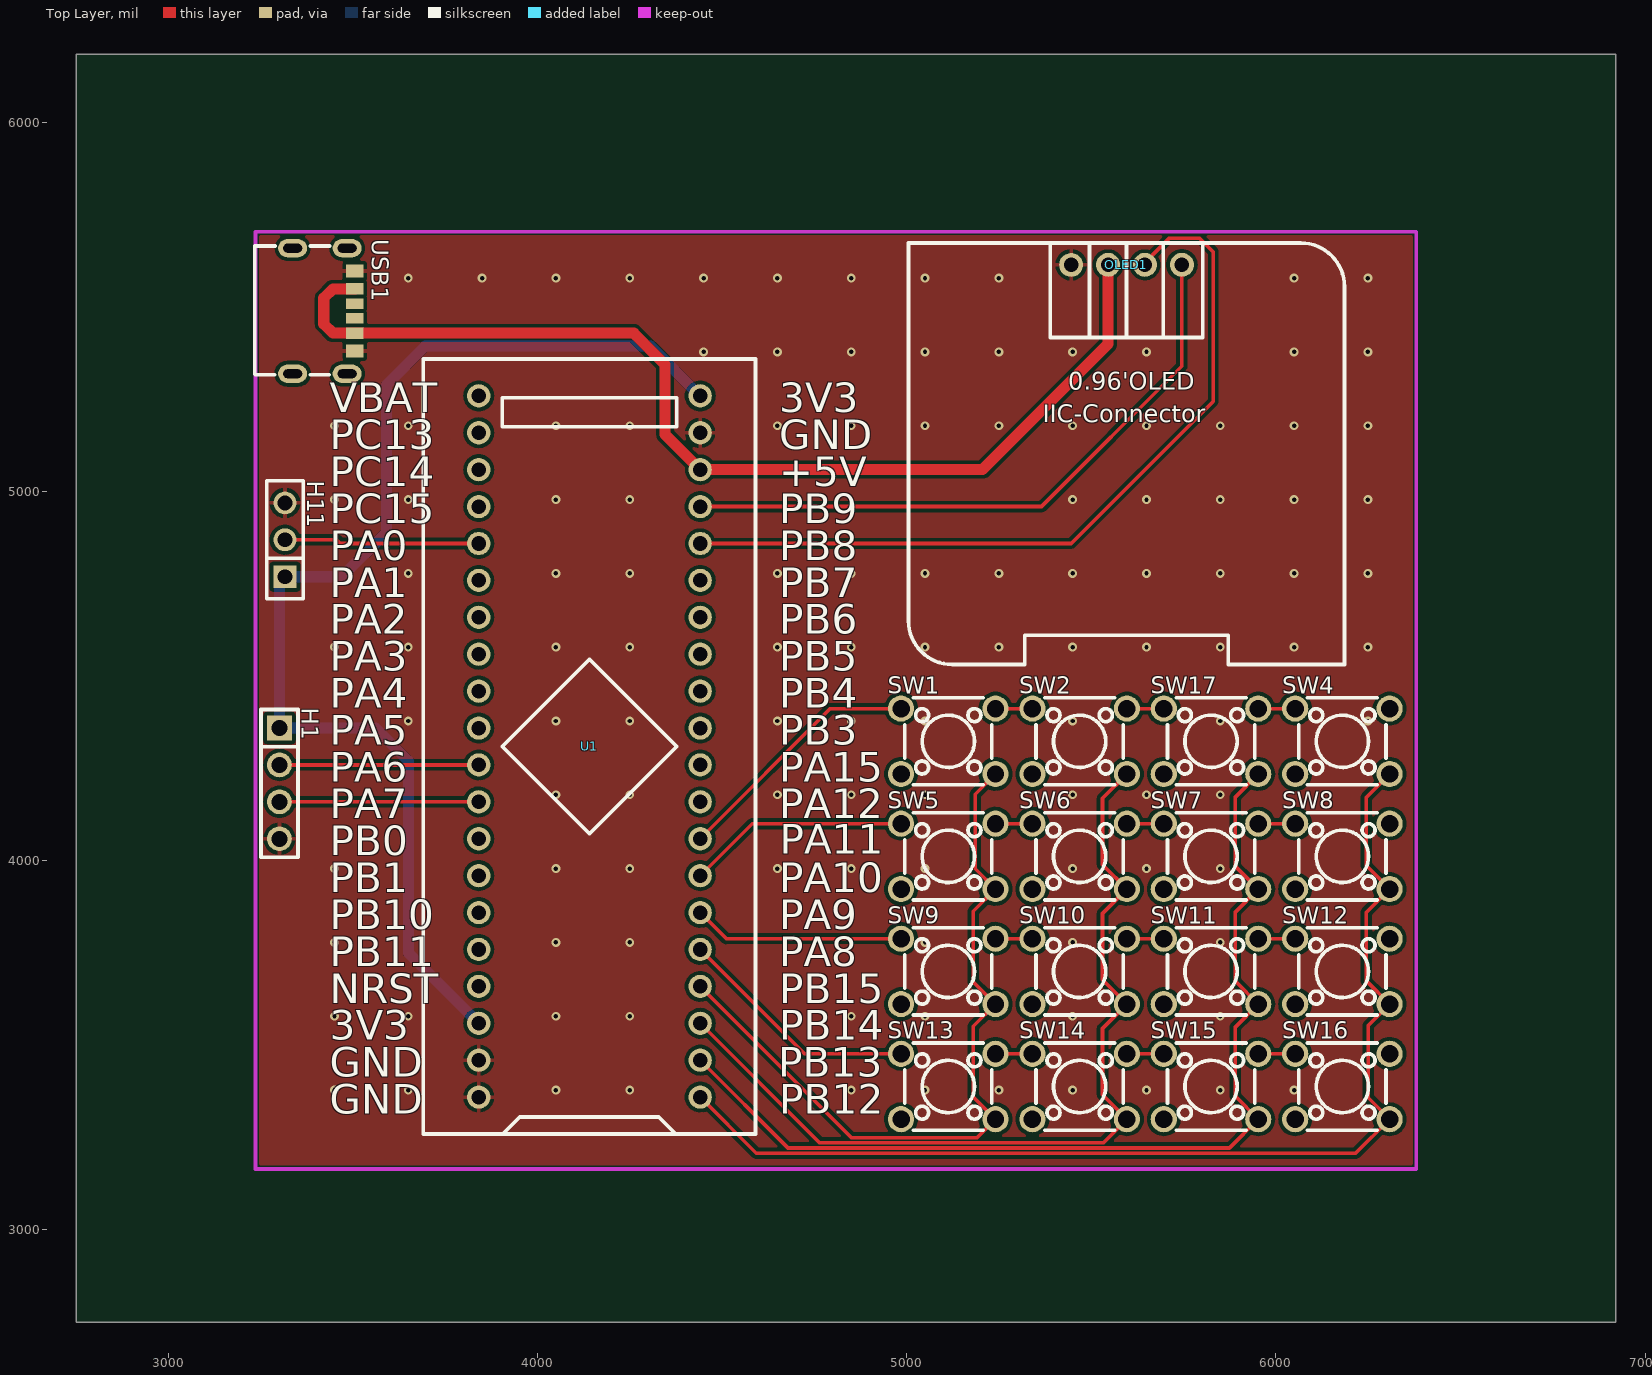
[diagram p0: Top Layer view]
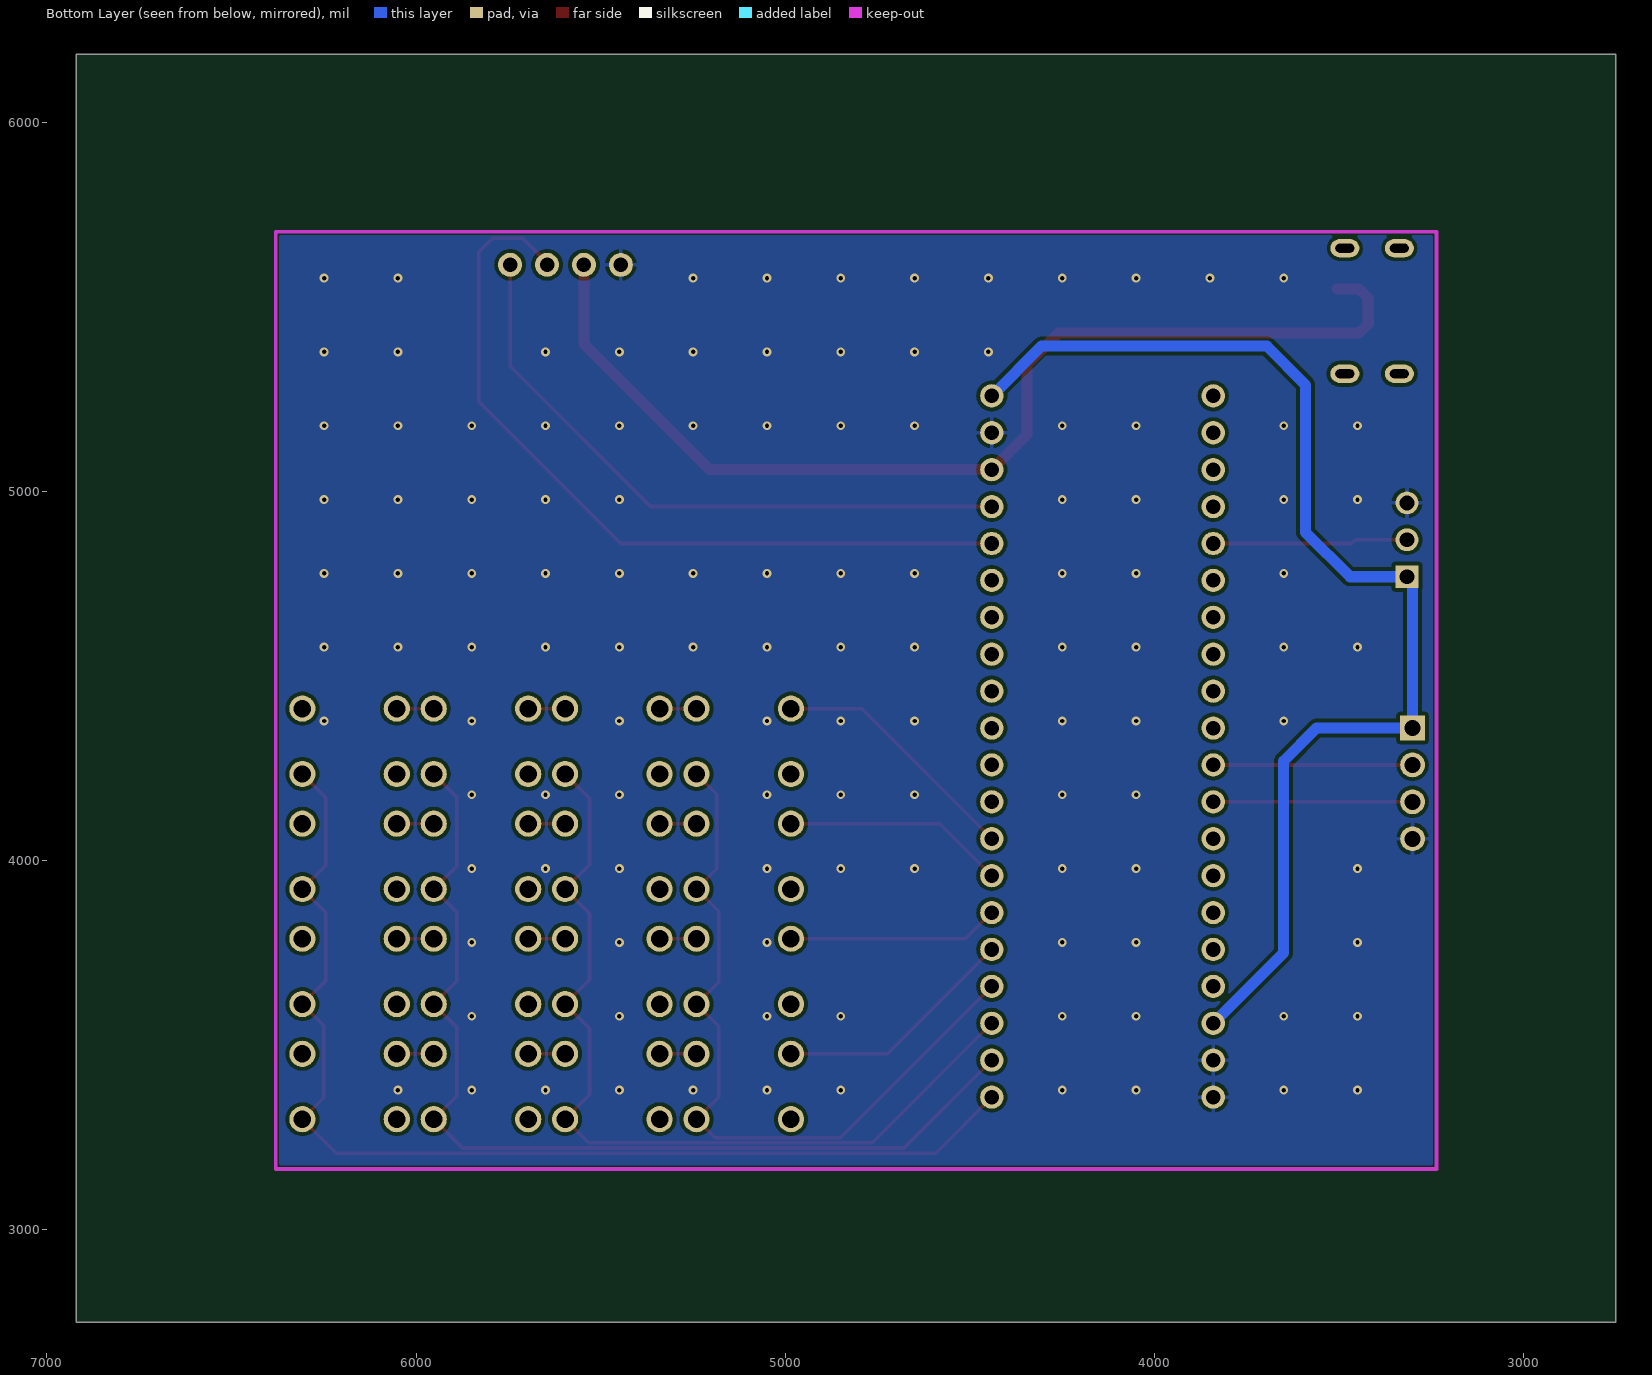
[diagram p1: Bottom Layer view, seen from below]
# Altium PCB MISC51803.pcbdoc
Units mil, origin at the board's own origin, x right, y up, seen from the top; angles counter-clockwise.
Board outline 4170 x 3435 mil, 2 copper layers (Top Layer, Bottom Layer), stack 62.206 mil thick; 21 components, 49 nets, 125 pads, 118 vias.

## Layer stack, top to bottom
Top Solder Mask Layer: solder mask 0.394, Dk 3.3
Top Layer: signal copper 1.379
Dielectric1: surface 59.449, FR4, Dk 4.5
Bottom Layer: signal copper 1.378
Bottom Solder Mask Layer: solder mask 0.394, Dk 3.3

## Board outline
6920,2750 2750,2750 2750,6185 6920,6185

## Design rules (kind name [scope] priority, off if disabled: settings)
BoardOutlineClearance copperThickness2oz_1 [All] p2 off: genericclearance=7.99 ignorepadtopadclearanceinfootprint=FALSE except(0: Arc-SplitContinuation Track-SplitContinuation SMDPad-SplitContinuation THPad-SplitContinuation Via-SplitContinuation Fill-SplitContinuation Region-SplitContinuation Poly-SplitContinuation Text-SplitContinuation Hole-SplitContinuation; 5.98: Arc-CutoutEdge SMDPad-CutoutEdge THPad-CutoutEdge Via-CutoutEdge Fill-CutoutEdge Region-CutoutEdge Text-CutoutEdge; 6.93: Hole-OutlineEdge Hole-CutoutEdge; 10: Poly-OutlineEdge Poly-CutoutEdge; 11.81: Arc-OutlineEdge Track-OutlineEdge SMDPad-OutlineEdge THPad-OutlineEdge Via-OutlineEdge Fill-OutlineEdge Region-OutlineEdge Text-OutlineEdge Track-CutoutEdge)
BoardOutlineClearance copperThickness1oz_1 [All] p4: genericclearance=4.02 ignorepadtopadclearanceinfootprint=FALSE except(0: Arc-SplitContinuation Track-SplitContinuation SMDPad-SplitContinuation THPad-SplitContinuation Via-SplitContinuation Fill-SplitContinuation Region-SplitContinuation Poly-SplitContinuation Text-SplitContinuation Hole-SplitContinuation; 6: SMDPad-CutoutEdge THPad-CutoutEdge Via-CutoutEdge Fill-CutoutEdge Region-CutoutEdge Text-CutoutEdge; 6.93: Hole-OutlineEdge Hole-CutoutEdge; 10: Poly-OutlineEdge Poly-CutoutEdge; 11.8: Arc-OutlineEdge Track-OutlineEdge SMDPad-OutlineEdge THPad-OutlineEdge Via-OutlineEdge Fill-OutlineEdge Region-OutlineEdge Text-OutlineEdge; 11.81: Arc-CutoutEdge Track-CutoutEdge)
Clearance copperThickness2oz [All] p1 off: gap=7.99 ignorepadtopadclearanceinfootprint=FALSE except(5.98: SMDPad-Track SMDPad-SMDPad THPad-Track SMDPad-THPad THPad-THPad Track-Via SMDPad-Via THPad-Via Via-Via Fill-Track Region-Track Fill-SMDPad Region-SMDPad Fill-THPad Region-THPad Fill-Via Region-Via Fill-Fill Fill-Region Region-Region Arc-Track Arc-SMDPad Arc-THPad Arc-Via Fill-Arc Region-Arc Arc-Arc Text-Track SMDPad-Text Text-THPad Text-Via Fill-Text Region-Text Arc-Text Text-Text; 6.93: Hole-Track Hole-SMDPad Hole-THPad Hole-Via Fill-Hole Region-Hole Hole-Arc Hole-Text; 10: Poly-Track Poly-SMDPad Poly-THPad Poly-Via Poly-Fill Poly-Region Poly-Poly Poly-Arc Poly-Text Poly-Hole)
Clearance copperThickness1oz [All] p3: gap=4.02 ignorepadtopadclearanceinfootprint=FALSE except(5.98: SMDPad-Track SMDPad-SMDPad THPad-Track SMDPad-THPad THPad-THPad Track-Via SMDPad-Via THPad-Via Via-Via Fill-Track Region-Track Fill-SMDPad Region-SMDPad Fill-THPad Region-THPad Fill-Via Region-Via Fill-Fill Fill-Region Region-Region; 6: Arc-Track Arc-SMDPad Arc-THPad Arc-Via Fill-Arc Region-Arc Arc-Arc Text-Track SMDPad-Text Text-THPad Text-Via Fill-Text Region-Text Arc-Text Text-Text; 6.93: Hole-Track Hole-SMDPad Hole-THPad Hole-Via Fill-Hole Region-Hole Hole-Arc Hole-Text; 10: Poly-Track Poly-SMDPad Poly-THPad Poly-Via Poly-Fill Poly-Region Poly-Poly Poly-Arc Poly-Text Poly-Hole)
DiffPairsRouting differentialPair [All] p1: maxlimit=6 minlimit=6 mostfreqgap=6 toplayer_minwidth=5 toplayer_prefwidth=10 toplayer_maxwidth=100 toplayer_mingap=6 toplayer_prefgap=6 toplayer_maxgap=6 bottomlayer_minwidth=5 bottomlayer_prefwidth=10 bottomlayer_maxwidth=100 bottomlayer_mingap=6 bottomlayer_prefgap=6 bottomlayer_maxgap=6 maxuncoupledlength=10
HoleToHoleClearance otherClearance [All] p1: gap=11.81 allowstackedmicrovias=TRUE
Length netLength [All] p1: minlimit=0 maxlimit=0
MatchedLengths netLengthTolerance [All] p1: tolerance=1000
PasteMaskExpansion pasteMaskExpansion [All] p1: expansion=0
PlaneConnect innerPlane [All] p1: planeconnectstyle=Relief reliefexpansion=20 reliefentries=4 reliefconductorwidth=10 reliefairgap=10
PolygonConnect copperRegion [(InNet('GND'))] p1: connectstyle=Relief reliefconductorwidth=10 reliefentries=4 polygonreliefangle="90 Angle" airgapwidth=10 via.connectstyle=Relief via.reliefconductorwidth=10 via.reliefentries=4 via.polygonreliefangle="90 Angle" via.airgapwidth=10
RoutingVias viaSize [All] p1: holewidth=12.01 width=24.02 viastyle="Through Hole" minholewidth=11.81 minwidth=19.68 maxholewidth=248.03 maxwidth=393.7
SolderMaskExpansion solderMaskExpansion [IsVia] p1: expansion=-1000 istentingtop=TRUE
SolderMaskExpansion solderMaskExpansion [All] p2: expansion=2 istentingtop=FALSE
Width copperThickness2oz_2 [All] p1 off: maxlimit=100 minlimit=8 preferedwidth=10
Width copperThickness1oz_2 [All] p2: maxlimit=100 minlimit=5 preferedwidth=10

## Components (designator, comment, footprint, x,y, rotation, side; value= is the part's Value field where it differs from the comment)
H1 "" HDR-TH_4P-P2.54-V-M 3300,4210 r270 top
H11 "" HDR-TH_3P-P2.54-V-F 3315,4870 r90 top
OLED1 "" 0.96OLED_4P 5595,5615 r0 top
SW1 "KH-6X6X6H-TJ" SW-TH_4P-L6.0-W6.0-P4.50-LS6.5 5112.09,4324.04 r0 top
SW2 "KH-6X6X6H-TJ" SW-TH_4P-L6.0-W6.0-P4.50-LS6.5 5468.06,4324.04 r0 top
SW4 "KH-6X6X6H-TJ" SW-TH_4P-L6.0-W6.0-P4.50-LS6.5 6180,4324.04 r0 top
SW5 "KH-6X6X6H-TJ" SW-TH_4P-L6.0-W6.0-P4.50-LS6.5 5112.09,4012.26 r0 top
SW6 "KH-6X6X6H-TJ" SW-TH_4P-L6.0-W6.0-P4.50-LS6.5 5468.06,4012.26 r0 top
SW7 "KH-6X6X6H-TJ" SW-TH_4P-L6.0-W6.0-P4.50-LS6.5 5824.03,4012.26 r0 top
SW8 "KH-6X6X6H-TJ" SW-TH_4P-L6.0-W6.0-P4.50-LS6.5 6180,4012.26 r0 top
SW9 "KH-6X6X6H-TJ" SW-TH_4P-L6.0-W6.0-P4.50-LS6.5 5112.09,3700.49 r0 top
SW10 "KH-6X6X6H-TJ" SW-TH_4P-L6.0-W6.0-P4.50-LS6.5 5468.06,3700.49 r0 top
SW11 "KH-6X6X6H-TJ" SW-TH_4P-L6.0-W6.0-P4.50-LS6.5 5824.03,3700.49 r0 top
SW12 "KH-6X6X6H-TJ" SW-TH_4P-L6.0-W6.0-P4.50-LS6.5 6180,3700.49 r0 top
SW13 "KH-6X6X6H-TJ" SW-TH_4P-L6.0-W6.0-P4.50-LS6.5 5112.09,3388.72 r0 top
SW14 "KH-6X6X6H-TJ" SW-TH_4P-L6.0-W6.0-P4.50-LS6.5 5468.06,3388.72 r0 top
SW15 "KH-6X6X6H-TJ" SW-TH_4P-L6.0-W6.0-P4.50-LS6.5 5824.03,3388.72 r0 top
SW16 "KH-6X6X6H-TJ" SW-TH_4P-L6.0-W6.0-P4.50-LS6.5 6180,3388.72 r0 top
SW17 "KH-6X6X6H-TJ" SW-TH_4P-L6.0-W6.0-P4.50-LS6.5 5824.03,4324.04 r0 top
U1 "STM32F103C8T6-Card" CONN-TH_L53.3-W22.9_STM32F103C8T6-CARD 4140,4310 r90 top
USB1 "" "USB_ TYPE-C-6P" 3420,5495 r270 top

## Footprints (in the part's own frame and the unit in brackets; to place one, negate y for a bottom-side part, rotate by r counter-clockwise, add the part's x,y. Pads: shape width x height; smd on the part's side, far side on the other; paste and mask are expansions set on the pad)
0.96OLED_4P [mm]
  round 1.65 hole 1 copper offset 0,0: 1(-3.81,-0.001) 2(-1.27,0.002) 3(1.27,0.002) 4(3.81,0.002)
  silkscreen extent -15,-27.5 15,1.5
CONN-TH_L53.3-W22.9_STM32F103C8T6-CARD [mm]
  round 1.6 hole 1: 1(-24.13,-7.62) 2(-21.59,-7.62) 3(-19.05,-7.62) 4(-16.51,-7.62) 5(-13.97,-7.62) 6(-11.43,-7.62) 7(-8.89,-7.62) 8(-6.35,-7.62) 9(-3.81,-7.62) 10(-1.27,-7.62) 11(1.27,-7.62) 12(3.81,-7.62) 13(6.35,-7.62) 14(8.89,-7.62) 15(11.43,-7.62) 16(13.97,-7.62) 17(16.51,-7.62) 18(19.05,-7.62) 19(21.59,-7.62) 20(24.13,-7.62) 21(24.13,7.62) 22(21.59,7.62) 23(19.05,7.62) 24(16.51,7.62) 25(13.97,7.62) 26(11.43,7.62) 27(8.89,7.62) 28(6.35,7.62) 29(3.81,7.62) 30(1.27,7.62) 31(-1.27,7.62) 32(-3.81,7.62) 33(-6.35,7.62) 34(-8.89,7.62) 35(-11.43,7.62) 36(-13.97,7.62) 37(-16.51,7.62) 38(-19.05,7.62) 39(-21.59,7.62) 40(-24.13,7.62)
  silkscreen extent -26.67,-11.43 26.67,11.43
HDR-TH_3P-P2.54-V-F [mil]
  rect 62x62 hole 40.16: 1(-100,0)
  round 62 hole 40.16: 2(0,0) 3(100,0)
  silkscreen extent -160,-49 160,49
HDR-TH_4P-P2.54-V-M [mm]
  rect 1.7x1.7 hole 1.1: 1(-3.81,0)
  round 1.7 hole 1.1: 2(-1.27,0) 3(1.27,0) 4(3.81,0)
  silkscreen extent -5.08,-1.27 5.08,1.27
SW-TH_4P-L6.0-W6.0-P4.50-LS6.5 [mm]
  round 1.8 hole 1.2: 1(-3.25,2.25) 2(3.25,2.25) 3(-3.25,-2.25) 4(3.25,-2.25)
  silkscreen extent -3,-3 3,3
"USB_ TYPE-C-6P" [mm]
  oval 1.25x2 hole 0.6 slot 1.3 at 90 deg paste+0 mask+0.05: 7(-4.193,1.611) 8(4.447,1.611) 9(-4.193,-2.139) 10(4.447,-2.139)
  rect 0.7x1.2 smd paste-100 mask+0.05: A5(-0.373,2.139) B5(0.627,2.139)
  rect 0.8x1.2 smd paste-100 mask+0.05: A9(1.647,2.139) B9(-1.393,2.139)
  rect 0.9x1.2 smd paste-100 mask+0.05: A12(2.877,2.139) B12(-2.623,2.139)
  silkscreen extent -4.34,-4.75 4.52,0.39

## Via types
v1: diameter 24.02, hole 12, Top Layer to Bottom Layer, 118 vias

## Nets (pads, with @x,y where several pads share a name; then routed paths per layer and width w, separated by ;. In a path a pad name is that pad's centre, name@x,y a point inside that pad or via, vN(x,y) a via of type N, cw(c..) or ccw(c..) an arc to the next point about the centre after c; other vN are vias at no path point)
$1N9: SW9.2 SW10.1 | length 100.1
  Top Layer w10: SW9.2 SW10.1
$1N10: SW13.2 SW14.1 | length 100.1
  Top Layer w10: SW13.2 SW14.1
$1N11: SW15.2 SW16.1 | length 100.1
  Top Layer w10: SW15.2 SW16.1
$1N12: SW14.2 SW15.1 | length 100.1
  Top Layer w10: SW14.2 SW15.1
$1N13: SW11.2 SW12.1 | length 100.1
  Top Layer w10: SW11.2 SW12.1
$1N14: SW10.2 SW11.1 | length 100.1
  Top Layer w10: SW10.2 SW11.1
$1N15: SW7.2 SW8.1 | length 100.1
  Top Layer w10: SW7.2 SW8.1
$1N16: SW5.2 SW6.1 | length 100.1
  Top Layer w10: SW5.2 SW6.1
$1N17: SW6.2 SW7.1 | length 100.1
  Top Layer w10: SW6.2 SW7.1
$1N18: SW1.2 SW2.1 | length 100.1
  Top Layer w10: SW1.2 SW2.1
$1N19: SW2.2 SW17.1 | length 100.1
  Top Layer w10: SW2.2 SW17.1
$1N20: SW4.1 SW17.2 | length 100.1
  Top Layer w10: SW17.2 SW4.1
+5V: OLED1.2 U1.18 USB1.A9 USB1.B9 | length 2920.3
  Top Layer w30: USB1.B9 3444.84,5549.84 3420,5525 3420,5455 3444.84,5430.16 USB1.A9 4259.84,5430.16 4345,5345 4345,5155 U1.18 5205,5060 5545,5400 OLED1.2@5545,5615.05
GND: H1.4 H11.3 OLED1.1 U1.19 U1.39 U1.40 USB1.A12 USB1.B12
  other v1: 3449.1,3379.1 3649.1,3379.1 4049.1,3379.1 4249.1,3379.1 4849.1,3379.1 5049.1,3379.1 5249.1,3379.1 5449.1,3379.1 5649.1,3379.1 5849.1,3379.1 6049.1,3379.1 3449.1,3579.1 3649.1,3579.1 4049.1,3579.1 4249.1,3579.1 4849.1,3579.1 5049.1,3579.1 5449.1,3579.1 5849.1,3579.1 3449.1,3779.1 4049.1,3779.1 4249.1,3779.1 5049.1,3779.1 5449.1,3779.1 5849.1,3779.1 3449.1,3979.1 4049.1,3979.1 4249.1,3979.1 4649.1,3979.1 4849.1,3979.1 5049.1,3979.1 5449.1,3979.1 5649.1,3979.1 5849.1,3979.1 4049.1,4179.1 4249.1,4179.1 4649.1,4179.1 4849.1,4179.1 5049.1,4179.1 5449.1,4179.1 5649.1,4179.1 5849.1,4179.1 3649.1,4379.1 4049.1,4379.1 4249.1,4379.1 4649.1,4379.1 4849.1,4379.1 5049.1,4379.1 5449.1,4379.1 5849.1,4379.1 6249.1,4379.1 3449.1,4579.1 3649.1,4579.1 4049.1,4579.1 4249.1,4579.1 4649.1,4579.1 4849.1,4579.1 5049.1,4579.1 5249.1,4579.1 5449.1,4579.1 5649.1,4579.1 5849.1,4579.1 6049.1,4579.1 6249.1,4579.1 3649.1,4779.1 4049.1,4779.1 4249.1,4779.1 4649.1,4779.1 4849.1,4779.1 5049.1,4779.1 5249.1,4779.1 5449.1,4779.1 5649.1,4779.1 5849.1,4779.1 6049.1,4779.1 6249.1,4779.1 3449.1,4979.1 3649.1,4979.1 4049.1,4979.1 4249.1,4979.1 5449.1,4979.1 5649.1,4979.1 5849.1,4979.1 6049.1,4979.1 6249.1,4979.1 3449.1,5179.1 3649.1,5179.1 4049.1,5179.1 4249.1,5179.1 4649.1,5179.1 4849.1,5179.1 5049.1,5179.1 5249.1,5179.1 5449.1,5179.1 5649.1,5179.1 5849.1,5179.1 6049.1,5179.1 6249.1,5179.1 4449.1,5379.1 4649.1,5379.1 4849.1,5379.1 5049.1,5379.1 5249.1,5379.1 5449.1,5379.1 5649.1,5379.1 6049.1,5379.1 6249.1,5379.1 3649.1,5579.1 3849.1,5579.1 4049.1,5579.1 4249.1,5579.1 4449.1,5579.1 4649.1,5579.1 4849.1,5579.1 5049.1,5579.1 5249.1,5579.1 6049.1,5579.1 6249.1,5579.1
NRST: U1.37
PA0: H11.2 U1.25 | length 529.1
  Top Layer w10: H11.2 3455,4870 3465,4860 U1.25
PA1: U1.26
PA2: U1.27
PA3: U1.28
PA4: U1.29
PA5: U1.30
PA6: H1.2 U1.31 | length 540
  Top Layer w10: H1.2 U1.31
PA7: H1.3 U1.32 | length 540
  Top Layer w10: H1.3 U1.32
PA8: SW13.1 U1.5 | length 661.2
  Top Layer w10: U1.5 4722.7,3477.3 SW13.1
PA9: SW9.1 U1.6 | length 573.5
  Top Layer w10: U1.6 4510.93,3789.07 SW9.1
PA10: SW5.1 U1.7 | length 602.5
  Top Layer w10: U1.7 4580.84,4100.84 SW5.1
PA11: SW1.1 U1.8 | length 690.2
  Top Layer w10: U1.8 4792.61,4412.62 SW1.1
PA12: U1.9
PA15: U1.10
PB0: U1.33
PB1: U1.34
PB3: U1.11
PB4: U1.12
PB5: U1.13
PB6: U1.14
PB7: U1.15
PB8: OLED1.3 U1.16 | length 2188.2
  Top Layer w10: U1.16 5445,4860 5830,5245 5830,5650 5793.33,5686.67 5710,5686.67 5645,5621.67 OLED1.3@5645,5615.05
PB9: OLED1.4 U1.17 | length 1737.5
  Top Layer w10: U1.17 5365,4960 5745,5340 OLED1.4@5745,5615.05
PB10: U1.35
PB11: U1.36
PB12: SW4.4 SW8.4 SW12.4 SW16.4 U1.1 | length 3056.7
  Top Layer w10: U1.1 4592.05,3207.95 6215.76,3207.95 SW16.4 6250,3358.09 6250,3553.97 SW12.4 6245,3674.86 6245,3860.74 SW8.4 6245,3986.63 6245,4172.51 SW4.4
PB13: SW7.4 SW11.4 SW15.4 SW17.4 U1.2 | length 2732.7
  Top Layer w10: U1.2 4678.03,3221.97 5873.81,3221.97 SW15.4 5890,3362.12 5890,3549.93 SW11.4 5890,3673.89 5890,3861.71 SW7.4 5951.32,3923.68 5890,3985 5890,4173.48 SW17.4
PB14: SW2.4 SW6.4 SW10.4 SW14.4 U1.3 | length 2416.2
  Top Layer w10: U1.3 4764.02,3235.98 5531.86,3235.98 SW14.4 5530,3366.15 5530,3545.9 SW10.4 5530,3677.92 5530,3857.67 SW6.4 5530,3989.7 5530,4169.45 SW2.4
PB15: SW1.4 SW5.4 SW9.4 SW13.4 U1.4 | length 2071
  Top Layer w10: U1.4 4850,3250 5189.9,3250 SW13.4 5180,3360.18 5180,3551.87 SW9.4 5180,3671.96 5180,3863.64 SW5.4 5185,3978.73 5185,4180.41 SW1.4
PC13: U1.22
PC14: U1.23
PC15: U1.24
VBAT: U1.21
VCC: H1.1 H11.1 U1.20 U1.38 | length 3266.3
  Bottom Layer w30: U1.38 3650,3750 3650,4270 3560,4360 H1.1 3300,4755 H11.1 3470,4770 3590,4890 3590,5290 3695,5395 4305,5395 U1.20
pads on no net: SW1.3 SW2.3 SW4.2 SW4.3 SW5.3 SW6.3 SW7.3 SW8.2 SW8.3 SW9.3 SW10.3 SW11.3 SW12.2 SW12.3 SW13.3 SW14.3 SW15.3 SW16.2 SW16.3 SW17.3 USB1.7 USB1.8 USB1.9 USB1.10 USB1.A5 USB1.B5

## Polygon pours and split planes (outlines as drawn)
GND on Top Layer (solid, remove dead copper, pour order 0): 3065,5930 3065,3000 6670,3000 6670,5930
GND on Bottom Layer (solid, remove dead copper, pour order 2): 3000,5935 3000,3035 6600,3035 6600,5935

## Keep-outs
Board Outline Layer:
  lines w10: 3235,3165 3235,5705 6380,5705 6380,3165 3235,3165

## Silkscreen, mask and mechanical layers (free items; w line width, h text height)
Top Silkscreen Layer:
  text "VBAT" at 3435.95,5215 h80
  text "3V3" at 4654.16,5215 h80
  text "PC13" at 3435.95,5115 h80
  text "GND" at 4654.16,5115 h80
  text "PC14" at 3435.95,5015 h80
  text "+5V" at 4654.16,5015 h80
  text "PC15" at 3435.95,4915 h80
  text "PB9" at 4654.16,4915 h80
  text "PA0" at 3435.95,4815 h80
  text "PB8" at 4654.16,4815 h80
  text "PA1" at 3435.95,4715 h80
  text "PB7" at 4654.16,4715 h80
  text "PA2" at 3435.95,4615 h80
  text "PB6" at 4654.16,4615 h80
  text "PA3" at 3435.95,4515 h80
  text "PB5" at 4654.16,4515 h80
  text "PA4" at 3435.95,4415 h80
  text "PB4" at 4654.16,4415 h80
  text "PA5" at 3435.95,4315 h80
  text "PB3" at 4654.16,4315 h80
  text "PA6" at 3435.95,4215 h80
  text "PA15" at 4654.16,4215 h80
  text "PA7" at 3435.95,4115 h80
  text "PA12" at 4654.16,4115 h80
  text "PA11" at 4655.95,4020 h80
  text "PB0" at 3435.95,4015 h80
  text "PB1" at 3435.95,3915 h80
  text "PA10" at 4654.16,3915 h80
  text "PB10" at 3435.95,3815 h80
  text "PA9" at 4654.16,3815 h80
  text "PB11" at 3435.95,3715 h80
  text "PA8" at 4654.16,3715 h80
  text "NRST" at 3435.95,3615 h80
  text "PB15" at 4654.16,3615 h80
  text "3V3" at 3435.95,3515 h80
  text "PB14" at 4654.16,3515 h80
  text "GND" at 3435.95,3415 h80
  text "PB13" at 4650.95,3415 h80
  text "GND" at 3435.95,3315 h80
  text "PB12" at 4654.16,3315 h80